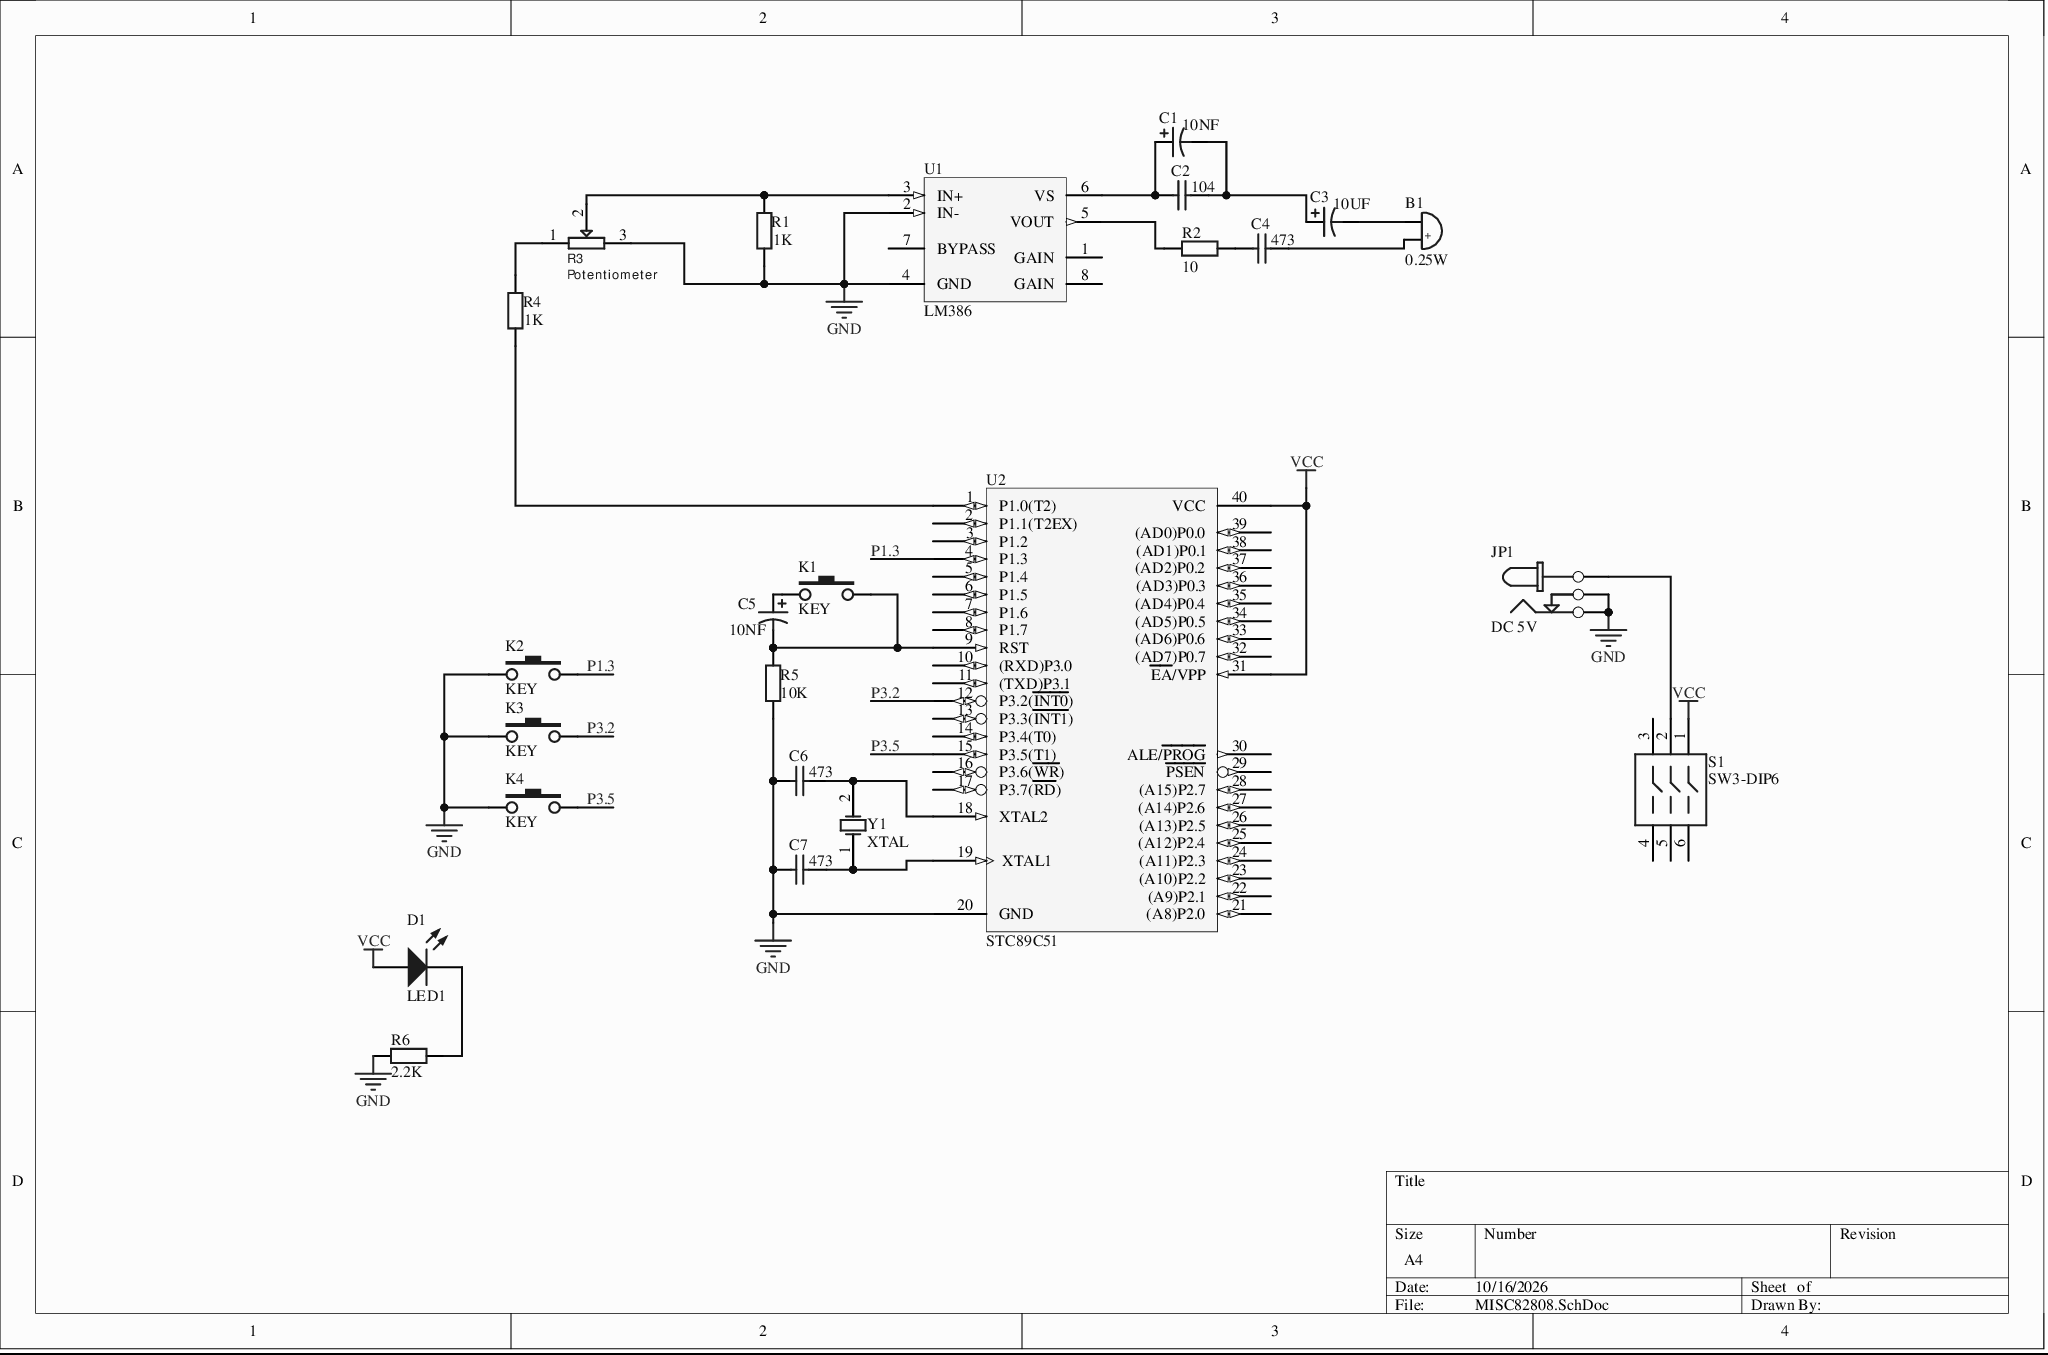
[diagram p0: MISC82808.SchDoc]
# Altium project MISC82808-7.PrjPcb
1 sheet, 24 parts. Net scope: global (net labels, ports and power ports of the same name join across sheets).
Board file: MISC82808.PcbDoc

## Sheet MISC82808.SchDoc
size A4

### Parts
B1  0.25W  [BEEP 5x9x5.5]
C1  value 10NF  [RB7.6-15]  (hidden comment: Cap Pol1)
C2  value 104  [RAD-0.3]  (hidden comment: Cap)
C3  value 10UF  [RB7.6-15]  (hidden comment: Cap Pol1)
C4  value 473  [RAD-0.3]  (hidden comment: Cap)
C5  value 10NF  [RB7.6-15]  (hidden comment: Cap Pol1)
C6  value 473  [RAD-0.3]  (hidden comment: Cap)
C7  value 473  [RAD-0.3]  (hidden comment: Cap)
D1  LED1  [LED-1]
JP1  DC 5V  [DC POWER JACK1]
K1  KEY  [DIP-3X6X4.3]
K2  KEY  [DIP-3X6X4.3]
K3  KEY  [DIP-3X6X4.3]
K4  KEY  [DIP-3X6X4.3]
R1  value 1K  [AXIAL-0.4]  (hidden comment: Res2)
R2  value 10  [AXIAL-0.4]  (hidden comment: Res2)
R3  Potentiometer  [滑动变阻器]
R4  value 1K  [AXIAL-0.4]  (hidden comment: Res2)
R5  value 10K  [AXIAL-0.4]  (hidden comment: Res2)
R6  value 2.2K  [AXIAL-0.4]  (hidden comment: Res2)
S1  SW3-DIP6  [DIP-Switch3]
U1  LM386  [M08A_N]
U2  STC89C51  [DIP40]
Y1  XTAL  [R38]

### Nets
GND: C6.1 C7.1 JP1.2(B) JP1.3(C) K2.1 K3.1 K4.1 R1.1 R3.3 R5.1 R6.2 U1.2(IN-) U1.4(GND) U2.20(GND)
VCC: D1.1(A) S1.1(A1) U2.31(~{EA}/VPP) U2.40(VCC)
P1.3: K2.3 U2.4(P1.3)
P3.2: K3.3 U2.12(P3.2(~{INT0}))
P3.5: K4.3 U2.15(P3.5(T1))
NetB1_1: B1.1 C4.2
NetB1_2: B1.2 C3.2
NetC1_1: C1.1 C2.1 U1.6(VS)
NetC1_2: C1.2 C2.2 C3.1
NetC4_1: C4.1 R2.2
NetC5_1: C5.1 K1.1
NetC5_2: C5.2 K1.3 R5.2 U2.9(RST)
NetC6_2: C6.2 U2.18(XTAL2) Y1.2(OSC2)
NetC7_2: C7.2 U2.19(XTAL1) Y1.1(OSC1)
NetD1_2: D1.2(K) R6.1
NetJP1_1: JP1.1(A) S1.2(A2)
NetR1_2: R1.2 R3.2 U1.3(IN+)
NetR2_1: R2.1 U1.5(VOUT)
NetR3_1: R3.1 R4.2
NetR4_1: R4.1 U2.1(P1.0(T2))

Not connected (* = marked no-connect by the designer): S1 3(A3) 4(B3) 5(B2) 6(B1); U1 1(GAIN) 7(BYPASS) 8(GAIN); U2 2(P1.1(T2EX)) 3(P1.2) 5(P1.4) 6(P1.5) 7(P1.6) 8(P1.7) 10((RXD)P3.0) 11((TXD)P3.1) 13(P3.3(~{INT1})) 14(P3.4(T0)) 16(P3.6(~{WR})) 17(P3.7(~{RD})) 21((A8)P2.0) 22((A9)P2.1) 23((A10)P2.2) 24((A11)P2.3) 25((A12)P2.4) 26((A13)P2.5) 27((A14)P2.6) 28((A15)P2.7) 29(~{PSEN}) 30(ALE/~{PROG}) 32((AD7)P0.7) 33((AD6)P0.6) 34((AD5)P0.5) 35((AD4)P0.4) 36((AD3)P0.3) 37((AD2)P0.2) 38((AD1)P0.1) 39((AD0)P0.0)

### Library data of the parts
B1 = BEEP: Buzzer
C1 C3 C5 = Cap Pol1: Polarized Capacitor (Radial); Published: 8-Jun-2000; LatestRevisionDate: 17-Jul-2002; LatestRevisionNote: Re-released for DXP Platform.; PackageReference: RB7.6-15; PackageDescription: Polarized Capacitor (Radial); 2 Leads; Publisher: Altium Limited
C2 C4 C6 C7 = Cap: Capacitor; Published: 8-Jun-2000; LatestRevisionDate: 17-Jul-2002; LatestRevisionNote: Re-released for DXP Platform.; PackageReference: RAD-0.3; PackageDescription: Radial Cap, Thru-Hole; 2 Leads; 0.3 in Pin Spacing; Publisher: Altium Limited
D1 = LED1: Typical RED GaAs LED; Published: 8-Jun-2000; LatestRevisionDate: 08-Jul-2005; LatestRevisionNote: Mech Layer 1 removed.; PackageReference: LED-1; PackageDescription: LED; 2 Leads; Publisher: Altium Limited
JP1 = DC POWER JACK1: DC power jack
R1 R2 R4-R6 = Res2: Resistor; Published: 8-Jun-2000; LatestRevisionDate: 17-Jul-2002; LatestRevisionNote: Re-released for DXP Platform.; PackageReference: AXIAL-0.4; PackageDescription: Axial Device, Thru-Hole; 2 Leads; 0.4 in Pin Spacing; Publisher: Altium Limited
R3 = 滑动变阻器
U1 = LM386M-1: Low Voltage Audio Power Amplifier, 8-pin Narrow SOIC; Manufacturer: National Semiconductor; PackageTopMarking: NSZXTT*LM386*M-1; PowerWise: N; CompType: Audio IC; Published: 4-Dec-2008; DatasheetVersion: Aug-2000; PackageVersion: revM, May-2009; PackageReference: M08A; PackageDescription: SOIC Narrow, 4.9 x 3.9 x 1.45mm, 8 Lead, 1.27mm Pitch; Supplier 1: Farnell; Supplier Part Number 1: 9488324; PartNumber: LM386M-1; RoHS: N; PinCount: 8; Code_JEDEC: MS-012-AA; Code_IPC: SOIC127P600-8; ComponentLink1Description: LM386 Datasheet; ComponentLink1URL: http://www.national.com/ds/LM/LM386.pdf; ComponentLink2Description: LM386 Web Page; ComponentLink2URL: http://www.national.com/pf/LM/LM386.html; ComponentLink3Description: M08A Package Page; ComponentLink3URL: http://www.national.com/packaging/folders/m08a.html; Publisher: Altium Limited
Y1 = XTAL: Crystal Oscillator; Published: 8-Jun-2000; LatestRevisionDate: 17-Jul-2002; LatestRevisionNote: Re-released for DXP Platform.; PackageReference: R38; PackageDescription: Crystal, Thru-Hole; 2 Leads; Body 3.1 x 8.2 mm (Dia.xH); Publisher: Altium Limited